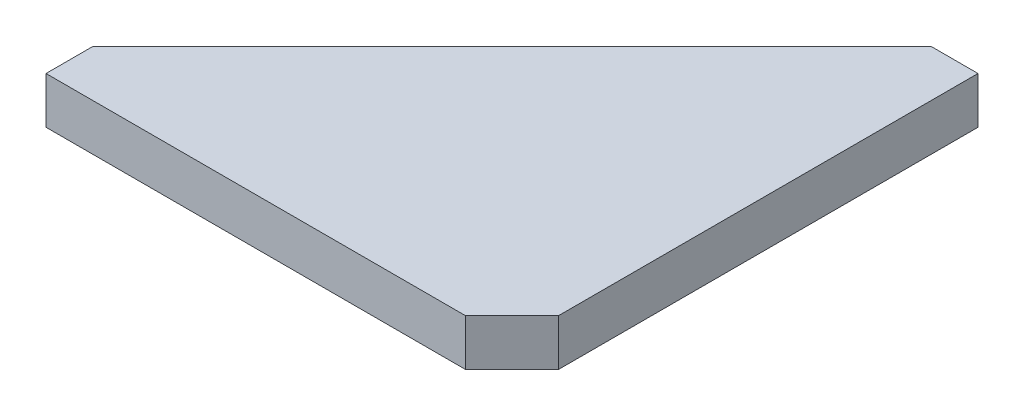
SolidWorks part; units mm, degrees
ref_plane "前视基准面" through (0, 0, 0) normal (0, 0, 1) x (1, 0, 0)
ref_plane "上视基准面" through (0, 0, 0) normal (0, 1, 0) x (1, 0, 0)
ref_plane "右视基准面" through (0, 0, 0) normal (1, 0, 0) x (0, 0, -1)
sketch "草图1" plane through (0, 0, 0) normal (0, 1, 0) x (1, 0, 0)
  line L0 (0, 0) -> (0, -180)
  line L1 (0, -180) -> (-20, -200)
  line L2 (-20, -200) -> (-200, -200)
  line L3 (-200, -200) -> (-200, -180)
  line L4 (-200, -180) -> (-20, 0)
  line L5 (-20, 0) -> (0, 0)
  point P3 (0, -181.1466)
  dimension "D1" = 20
  dimension "D2" = 200
  dimension "D3" = 200
  dimension "D4" = 20
  dimension "D5" = 45
  dimension "D6" = 20
extrude "凸台-拉伸1" add sketch "草图1" along normal blind 20
